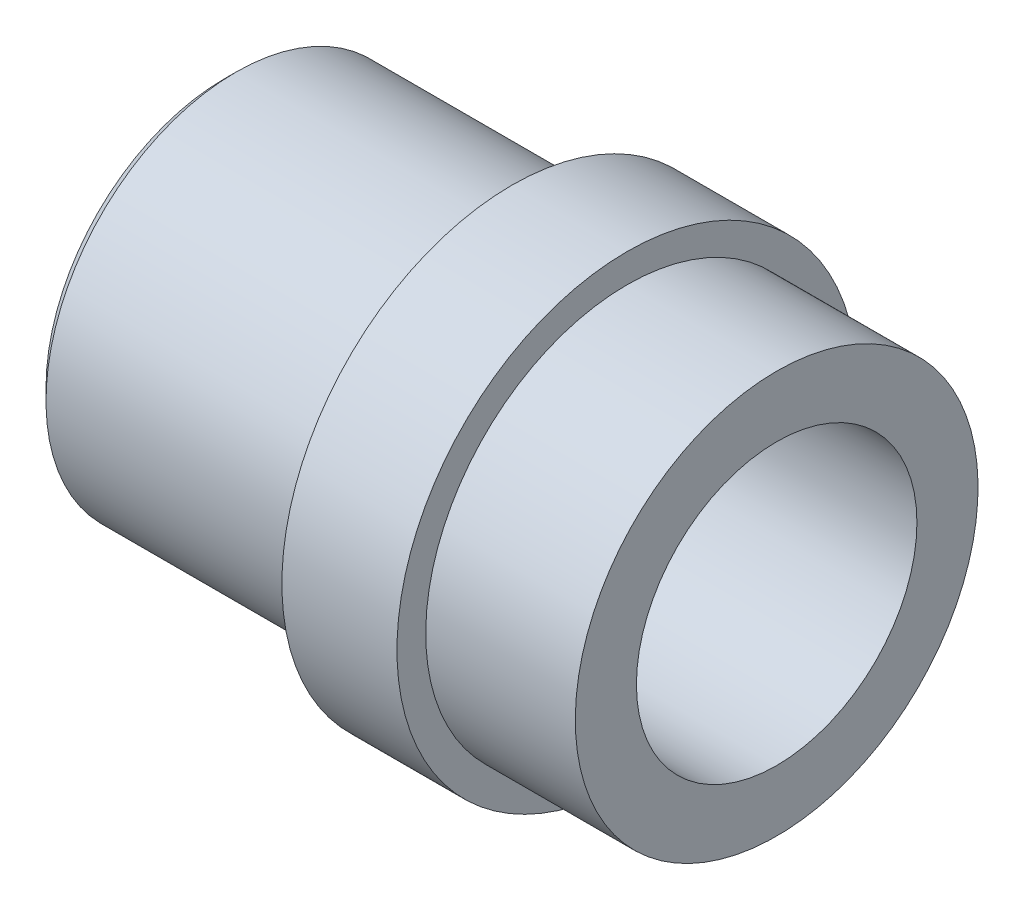
from build123d import *

# Parameters (mm, degrees)
SKETCH2_R          = 10.25
CUT_EXTRUDE1_DEPTH = 56.713553109
SKETCH4_R          = 12.188770661
CUT_EXTRUDE2_DEPTH = 20


with BuildPart() as part:
    # Sketch1 → Revolve1 (revolve)
    with BuildSketch(Plane.XY):
        Polygon((-48, 0), (-48, 15.5), (-47, 16.5), (-23, 16.5), (-23, 20), (-13, 20), (-13, 17.5), (0, 17.5), (0, 0), align=None)
    revolve(axis=Axis((0, 0, 0), (-1, 0, 0)))

    # Sketch2 → Cut-Extrude1 (cut, through all)
    with BuildSketch(Plane(origin=(0, 0, 0), x_dir=(0, 0, -1), z_dir=(1, 0, 0))):
        with Locations(Location((0, 0, 0), (0, 0, 90))):
            Circle(SKETCH2_R)
    extrude(amount=-CUT_EXTRUDE1_DEPTH, mode=Mode.SUBTRACT)

    # Sketch4 → Cut-Extrude2 (cut)
    with BuildSketch(Plane(origin=(0, 0, 0), x_dir=(0, 0, -1), z_dir=(1, 0, 0))):
        with Locations(Location((0, 0, 0), (0, 0, 90))):
            Circle(SKETCH4_R)
    extrude(amount=-CUT_EXTRUDE2_DEPTH, mode=Mode.SUBTRACT)


solid = part.part
